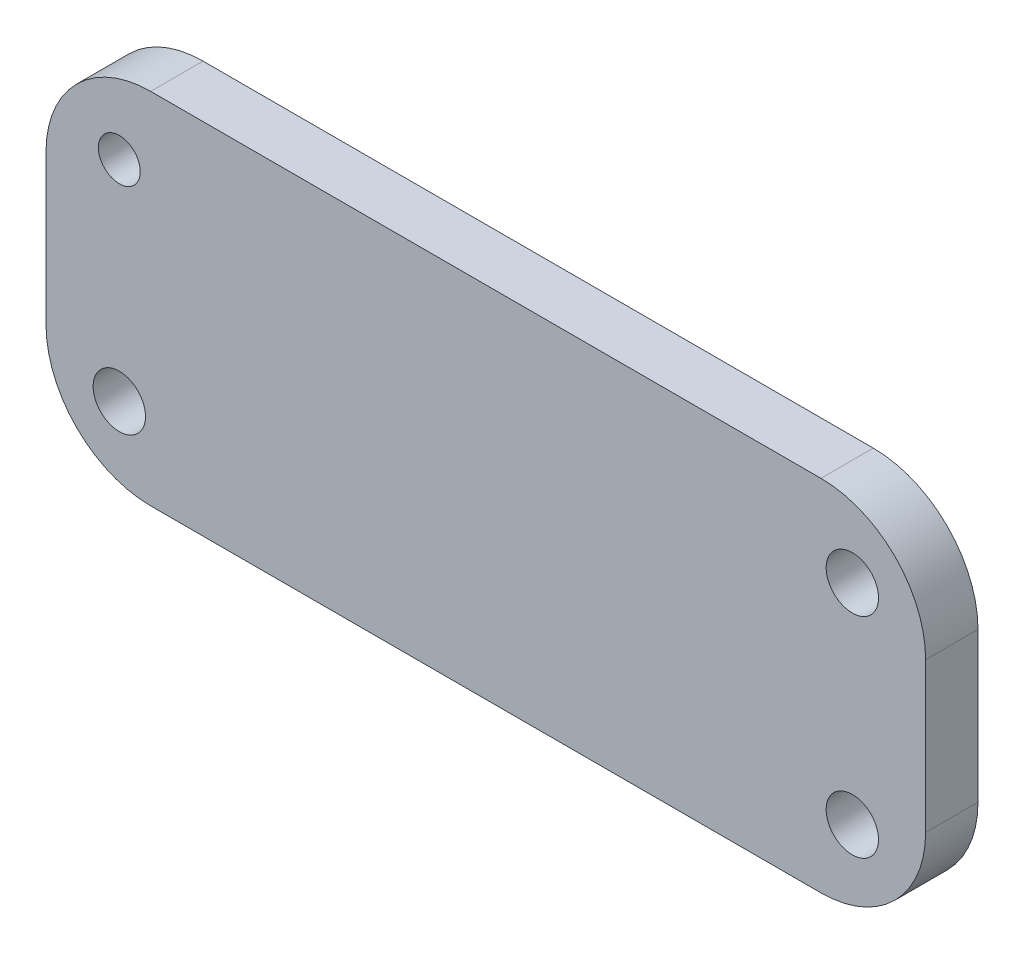
from build123d import *

# Parameters (mm, degrees)
SKETCH_1_W          = 168
SKETCH_1_H          = 68.565713714
EXTRUDE_1_DEPTH     = 10
SKETCH_2_R          = 4
SKETCH_2_R_2        = 5
CUT_EXTRUDE_1_DEPTH = 10
FILLET_1_R          = 20


with BuildPart() as part:
    # 草图1 → 凸台-拉伸1 (new body)
    with BuildSketch(Plane.XY):
        with Locations((0, -80)):
            Rectangle(SKETCH_1_W, SKETCH_1_H)
    extrude(amount=-EXTRUDE_1_DEPTH)

    # 草图2 → 切除-拉伸1 (cut)
    with BuildSketch(Plane.XY):
        with Locations((-70, -60)):
            Circle(SKETCH_2_R)
        with Locations((-70, -100)):
            Circle(SKETCH_2_R_2)
        with Locations((70, -60)):
            Circle(SKETCH_2_R_2)
        with Locations((70, -100)):
            Circle(SKETCH_2_R_2)
    extrude(amount=-CUT_EXTRUDE_1_DEPTH, mode=Mode.SUBTRACT)

    # 圆角1
    fillet_1_edges = [part.edges().sort_by_distance(p)[0] for p in [
        (-84, -45.717143143, -5),
        (84, -45.717143143, -5),
        (84, -114.282856857, -5),
        (-84, -114.282856857, -5),
    ]]
    fillet(fillet_1_edges, radius=FILLET_1_R)


solid = part.part
